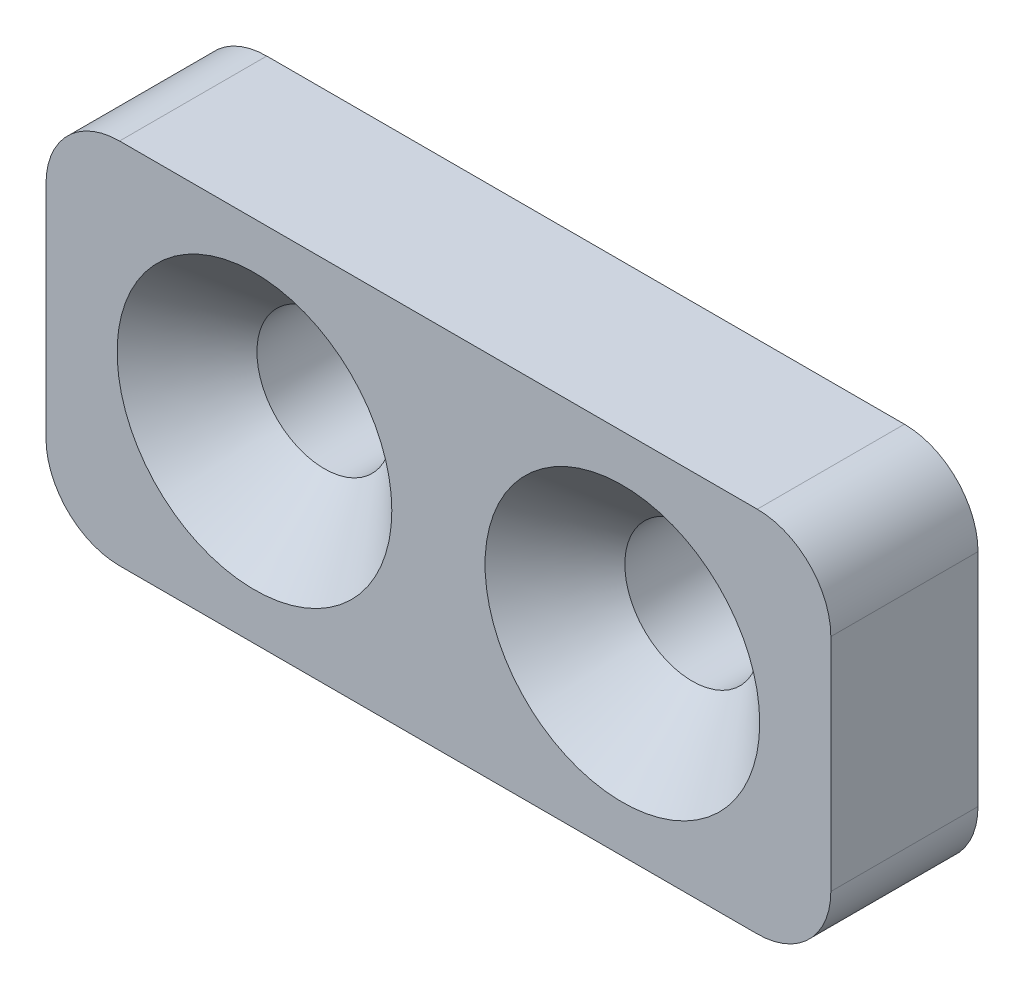
SolidWorks part; units mm, degrees
material "优力胶"
ref_plane "Front Plane" through (0, 0, 0) normal (0, 0, 1) x (1, 0, 0)
ref_plane "Top Plane" through (0, 0, 0) normal (0, 1, 0) x (1, 0, 0)
ref_plane "Right Plane" through (0, 0, 0) normal (1, 0, 0) x (0, 0, -1)
sketch "Sketch1" plane through (0, 0, 0) normal (0, 0, 1) x (1, 0, 0)
  line L1 (-16, -7.5) -> (16, -7.5)
  line L2 (-16, -7.5) -> (-16, 7.5)
  line L3 (-16, 7.5) -> (16, 7.5)
  line L4 (16, -7.5) -> (16, 7.5)
  line L5 (-16, -7.5) -> (16, 7.5) construction
  line L6 (-16, 7.5) -> (16, -7.5) construction
  point P0 (0, 0)
  dimension "D1" = 15
  dimension "D2" = 32
extrude "Boss-Extrude1" add sketch "Sketch1" along normal blind 6
hole_wizard "CSK for M5 Slotted raised CTSK head wood screws1" positions "Sketch2" profile "Sketch3" countersink size "M5" standard "GB"
sketch "Sketch2" plane through (0, 0, 6) normal (0, 0, 1) x (1, 0, 0)
  line L0 (0, 7.5) -> (0, -7.5) construction
  line L1 (16, 7.5) -> (-16, 7.5) construction
  line L2 (-16, -7.5) -> (16, -7.5) construction
  line L4 (-16, 0) -> (16, 0) construction
  line L5 (-16, 7.5) -> (-16, -7.5) construction
  line L6 (16, -7.5) -> (16, 7.5) construction
  point P20 (60, 0)
  point P22 (-60, 0)
  point P23 (-7.5, 0)
  point P25 (7.5, 0)
  dimension "D1" = 120
  dimension "D2" = 15
sketch "Sketch3" plane through (7.5, 0, 6) normal (1, 0, 0) x (0, -1, 0)
  line L0 (0, 0) -> (0, 14.0524)
  line L1 (0, 14.0524) -> (2.75, 12.4)
  line L2 (2.75, 12.4) -> (2.75, 2.85)
  line L3 (2.75, 2.85) -> (5.6, 0)
  line L5 (5.6, 0) -> (0, 0)
  line L6 (-2.75, 2.85) -> (-5.6, 0) construction
  line L10 (0, 14.0524) -> (-2.75, 12.4) construction
  line L11 (0, -6.35) -> (0, 107.95) construction
  dimension "孔直径" = 5.5
  dimension "孔深度" = 12.4
  dimension "近端锥形沉头孔直径" = 11.2
  dimension "近端锥形沉头孔角度" = 90
  dimension "导头角度" = 118
fillet "Fillet1" radius 3 4 edges at (16, -7.5, 3) (16, 7.5, 3) (-16, -7.5, 3) (-16, 7.5, 3)
